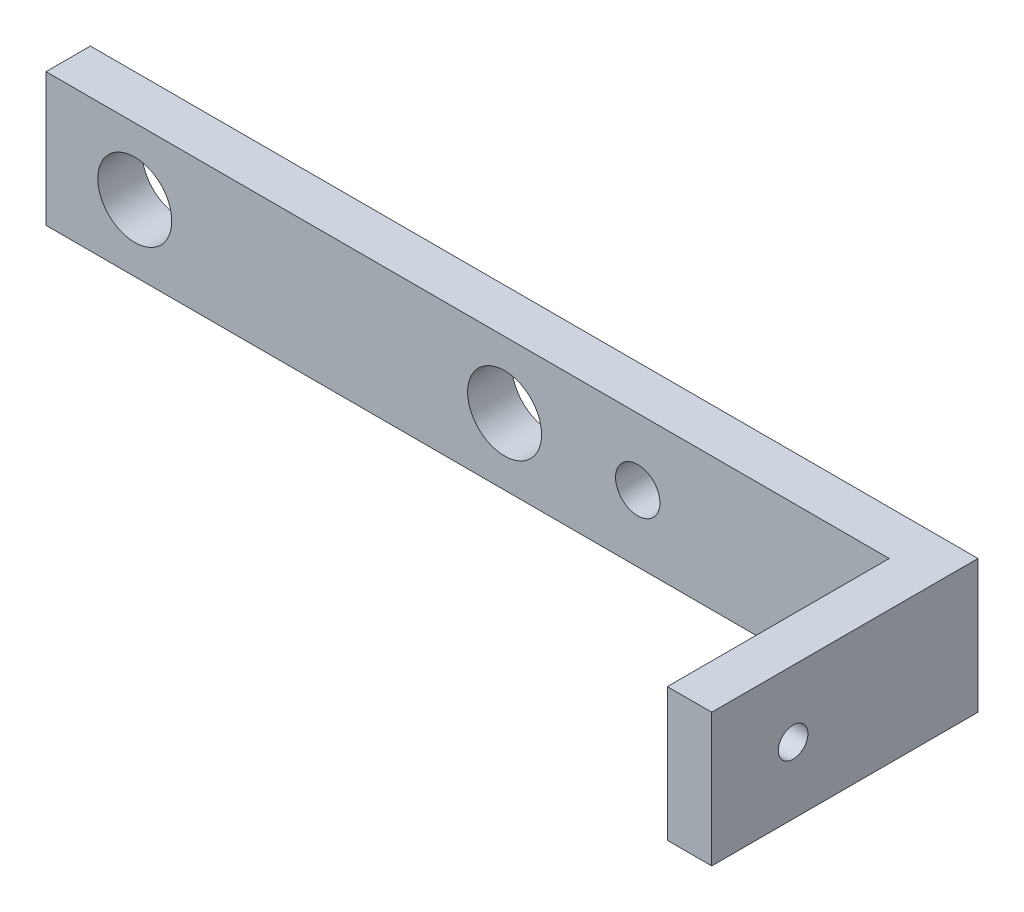
SolidWorks part; units mm, degrees
ref_plane "前视基准面" through (0, 0, 0) normal (0, 0, 1) x (1, 0, 0)
ref_plane "上视基准面" through (0, 0, 0) normal (0, 1, 0) x (1, 0, 0)
ref_plane "右视基准面" through (0, 0, 0) normal (1, 0, 0) x (0, 0, -1)
sketch "草图1" plane through (0, 0, 0) normal (0, 0, 1) x (1, 0, 0)
  line L1 (-47.5, -9) -> (47.5, -9)
  line L2 (-47.5, -9) -> (-47.5, 9)
  line L3 (-47.5, 9) -> (47.5, 9)
  line L4 (47.5, -9) -> (47.5, 9)
  line L5 (-47.5, -9) -> (47.5, 9) construction
  line L6 (-47.5, 9) -> (47.5, -9) construction
  point P0 (0, 0)
  dimension "D1" = 18
  dimension "D2" = 95
extrude "凸台-拉伸1" add sketch "草图1" along normal blind 6
sketch "草图2" plane through (0, 0, 6) normal (0, 0, 1) x (1, 0, 0)
  line L0 (14.5, 29.7699) -> (14.5, -28.1367) construction
  line L1 (-35.5, 29.7699) -> (-35.5, -29.7699) construction
  line L2 (47.5, -9) -> (47.5, 9) construction
  line L3 (-47.5, 0) -> (47.5, 0) construction
  line L4 (-47.5, 9) -> (-47.5, -9) construction
  circle A0 centre (-35.5, 0) radius 5
  circle A1 centre (14.5, 0) radius 5
  dimension "D3" = 10
  dimension "D4" = 10
  dimension "D1" = 33
  dimension "D2" = 50
extrude "切除-拉伸1" cut sketch "草图2" against normal blind 6
sketch "草图5" plane through (0, 0, 0) normal (0, 0, -1) x (-1, 0, 0)
  line L0 (-32.5, 21.0429) -> (-32.5, -19.2584) construction
  line L1 (-14.5, 0) -> (-33.9066, 0) construction
  circle A0 centre (-32.5, 0) radius 3
  dimension "D2" = 6
  dimension "D1" = 18
extrude "切除-拉伸3" cut sketch "草图5" against normal blind 10
sketch "草图6" plane through (47.5, 0, 0) normal (1, 0, 0) x (0, 0, -1)
  line L0 (-6, -9) -> (0, -9) construction
  line L1 (0, 9) -> (-6, 9)
  line L2 (0, 9) -> (0, -9)
  line L3 (0, -9) -> (-6, -9)
  line L4 (-6, 9) -> (-6, -9)
  dimension "D1" = 6
extrude "凸台-拉伸3" add sketch "草图6" along normal blind 25
sketch "草图7" plane through (0, 0, 6) normal (0, 0, 1) x (1, 0, 0)
  line L0 (-47.5, -9) -> (72.5, -9) construction
  line L1 (72.5, 9) -> (66.5, 9)
  line L2 (72.5, 9) -> (72.5, -9)
  line L3 (72.5, -9) -> (66.5, -9)
  line L4 (66.5, 9) -> (66.5, -9)
  dimension "D1" = 6
extrude "凸台-拉伸4" add sketch "草图7" along normal blind 30
sketch "草图8" plane through (72.5, 0, 0) normal (1, 0, 0) x (0, 0, -1)
  line L0 (0, -9) -> (0, 9) construction
  circle A0 centre (-25, 0) radius 2
  dimension "D1" = 4
  dimension "D2" = 25
extrude "切除-拉伸4" cut sketch "草图8" against normal blind 20
